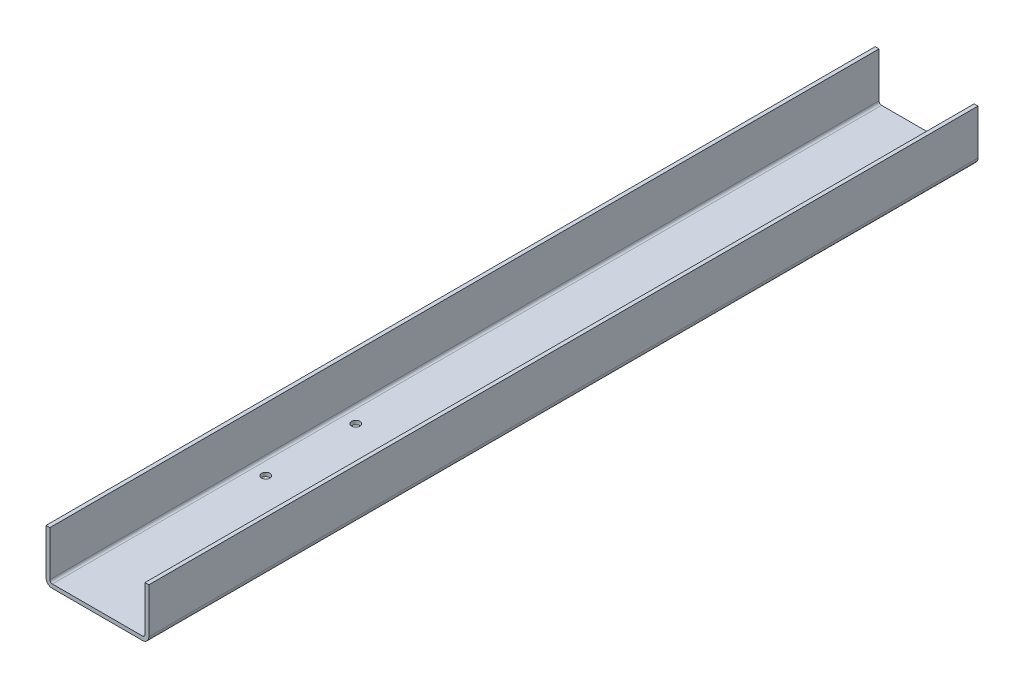
SolidWorks part; units mm, degrees
material "1023 Carbon Steel Plate (SS)"
ref_plane "Front Plane" through (0, 0, 0) normal (0, 0, 1) x (1, 0, 0)
ref_plane "Top Plane" through (0, 0, 0) normal (0, 1, 0) x (1, 0, 0)
ref_plane "Right Plane" through (0, 0, 0) normal (1, 0, 0) x (0, 0, -1)
sketch "Sketch1" plane through (0, 0, 0) normal (0, 0, 1) x (1, 0, 0)
  line L0 (0, 0) -> (0, -35)
  line L1 (5, -40) -> (75, -40)
  line L2 (80, -35) -> (80, 0)
  line L3 (3, 0) -> (3, -35)
  line L4 (5, -37) -> (75, -37)
  line L5 (77, -35) -> (77, 0)
  line L6 (3, 0) -> (0, 0)
  line L7 (80, 0) -> (77, 0)
  arc A0 (75, -40) -> (80, -35) centre (75, -35) ccw
  arc A1 (0, -35) -> (5, -40) centre (5, -35) ccw
  arc A2 (3, -35) -> (5, -37) centre (5, -35) ccw
  arc A3 (75, -37) -> (77, -35) centre (75, -35) ccw
  point P7 (80, -40)
  point P10 (0, -40)
  dimension "D4" = 5
  dimension "D1" = 80
  dimension "D2" = 40
  dimension "D3" = 40
  dimension "D5" = 3
extrude "Boss-Extrude1" add sketch "Sketch1" along normal blind 645 contours L7 L5 A3 L4 A2 L3 L6 L0 A1 L1 A0 L2
sketch "Sketch2" plane through (0, -40, 0) normal (0, -1, 0) x (1, 0, 0)
  line L0 (5, 645) -> (75, 645) construction
  line L1 (15, 419) -> (65, 419) construction
  line L2 (15, 419) -> (15, 489) construction
  line L3 (15, 489) -> (65, 489) construction
  line L4 (65, 419) -> (65, 489) construction
  line L5 (15, 419) -> (65, 489) construction
  line L6 (15, 489) -> (65, 419) construction
  circle A0 centre (15, 489) radius 3.25
  circle A1 centre (65, 489) radius 3.25
  circle A3 centre (15, 419) radius 3.25
  circle A4 centre (65, 419) radius 3.25
  point P0 (40, 454)
  point P7 (40, 489)
  point P8 (40, 645)
  dimension "D4" = 6.5
  dimension "D1" = 50
  dimension "D2" = 70
  dimension "D3" = 156
extrude "Cut-Extrude1" cut sketch "Sketch2" against normal blind 10
